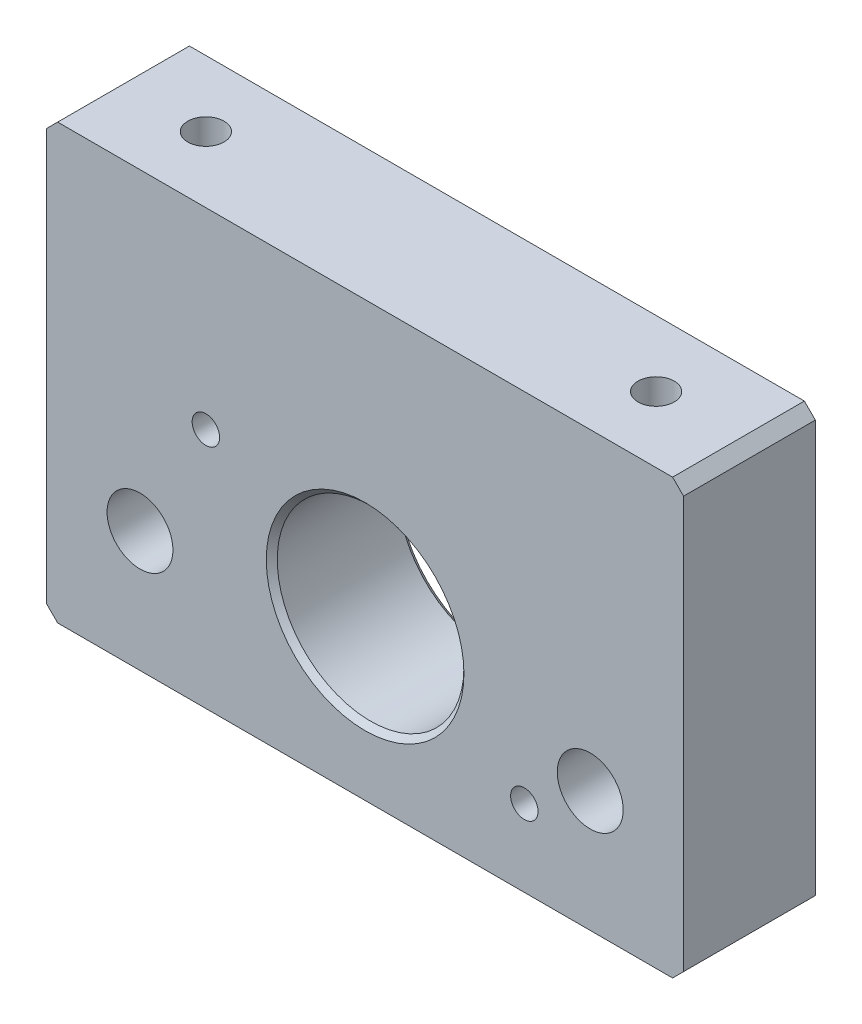
SolidWorks part; units mm, degrees
material "S45C"
ref_plane "Front Plane" through (0, 0, 0) normal (0, 0, 1) x (1, 0, 0)
ref_plane "Top Plane" through (0, 0, 0) normal (0, 1, 0) x (1, 0, 0)
ref_plane "Right Plane" through (0, 0, 0) normal (1, 0, 0) x (0, 0, -1)
sketch "Sketch1" plane through (0, 0, 0) normal (0, 0, 1) x (1, 0, 0)
  line L0 (-29, -8.75) -> (29, -8.75) construction
  line L1 (-29, 19.75) -> (29, 19.75)
  line L2 (-29, 19.75) -> (-29, -19.75)
  line L3 (-29, -19.75) -> (29, -19.75)
  line L4 (29, 19.75) -> (29, -19.75)
  line L5 (-29, 19.75) -> (29, -19.75) construction
  line L6 (-29, -19.75) -> (29, 19.75) construction
  line L7 (0, 19.75) -> (0, -19.75) construction
  circle A0 centre (0, -5.25) radius 8.5
  circle A1 centre (-20.5, -8.75) radius 3
  circle A2 centre (20.5, -8.75) radius 3
  point P0 (0, 0)
  dimension "D3" = 17
  dimension "D4" = 41
  dimension "D5" = 6
  dimension "D7" = 25
  dimension "D1" = 39.5
  dimension "D2" = 58
  dimension "D6" = 11
extrude "Boss-Extrude1" add sketch "Sketch1" along normal mid plane 12
hole_wizard "M3 Tapped Hole1" positions "Sketch3" profile "Sketch2" tap size "M3" standard "GB" end condition through all
sketch "Sketch3" plane through (0, 0, 6) normal (0, 0, 1) x (1, 0, 0)
  circle A0 centre (0, -5.25) radius 8.5 construction
  point P0 (-14.5, 2.25)
  point P1 (14.5, -12.75)
  dimension "D2" = 14.5
  dimension "D4" = 7.5
  dimension "D1" = 29
  dimension "D3" = 15
cosmetic thread "Hole thread1" parameters "D2"=3
cosmetic thread "Hole thread2" parameters "D2"=3
sketch "Sketch2" plane through (-14.5, 2.25, 6) normal (1, 0, 0) x (0, -1, 0)
  line L0 (0, 0) -> (0, 12)
  line L1 (0, 12) -> (1.25, 12)
  line L2 (1.25, 12) -> (1.25, 0)
  line L5 (1.25, 0) -> (0, 0)
  line L11 (0, -6.35) -> (0, 107.95) construction
  dimension "通孔螺纹孔钻头直径" = 2.5
  dimension "通孔螺纹孔钻头深度" = 12
hole_wizard "M4 Tapped Hole1" positions "Sketch5" profile "Sketch4" tap size "M4" standard "GB"
sketch "Sketch5" plane through (0, -19.75, 0) normal (0, -1, 0) x (1, 0, 0)
  line L0 (0, 6) -> (0, -6) construction
  line L1 (-29, 6) -> (29, 6) construction
  line L2 (-29, -6) -> (29, -6) construction
  point P0 (-20.5, 0)
  point P1 (20.5, 0)
  dimension "D1" = 41
cosmetic thread "Hole thread3" parameters "D1"=8, "D2"=4
cosmetic thread "Hole thread4" parameters "D1"=8, "D2"=4
sketch "Sketch4" plane through (-20.5, -19.75, 0) normal (1, 0, 0) x (0, 0, -1)
  line L0 (0, 0) -> (0, 11.0914)
  line L1 (0, 11.0914) -> (1.65, 10.1)
  line L2 (1.65, 10.1) -> (1.65, 0)
  line L5 (1.65, 0) -> (0, 0)
  line L10 (0, 11.0914) -> (-1.65, 10.1) construction
  line L11 (0, -6.35) -> (0, 107.95) construction
  dimension "螺纹孔钻头直径" = 3.3
  dimension "螺纹孔钻头深度" = 10.1
  dimension "导头角度" = 118
mirror "Mirror1" about plane through (0, 0, 0) normal (0, 1, 0) of "M4 Tapped Hole1"
chamfer "Chamfer1" distance 1 angle 45 4 edges at (29, 19.75, 0) (-29, 19.75, 0) (-29, -19.75, 0) (29, -19.75, 0)
chamfer "Chamfer2" distance 0.5 angle 45 2 edges at (8.5, -5.25, -6) (8.5, -5.25, 6)
